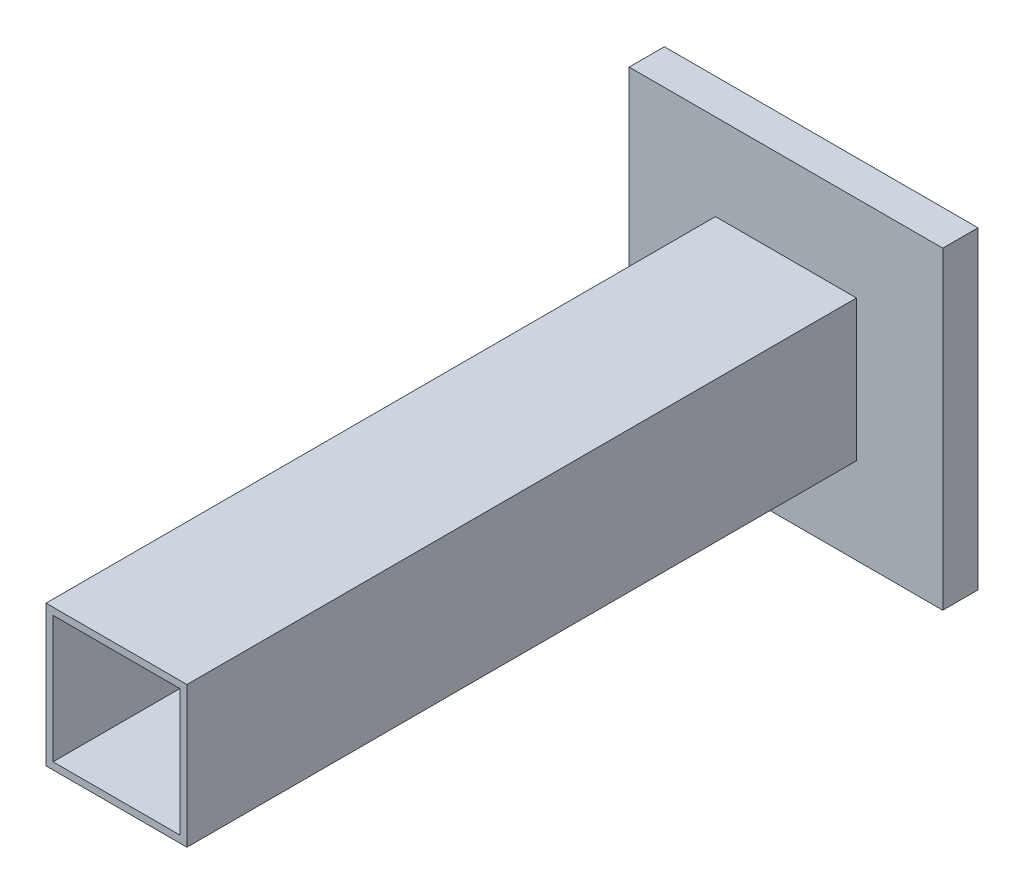
SolidWorks part; units mm, degrees
ref_plane "Front Plane" through (0, 0, 0) normal (0, 0, 1) x (1, 0, 0)
ref_plane "Top Plane" through (0, 0, 0) normal (0, 1, 0) x (1, 0, 0)
ref_plane "Right Plane" through (0, 0, 0) normal (1, 0, 0) x (0, 0, -1)
other "Configuration Table"
sketch "Sketch1" plane through (0, 0, 0) normal (0, 0, 1) x (1, 0, 0)
  line L1 (-222.5, 222.5) -> (222.5, 222.5)
  line L2 (-222.5, 222.5) -> (-222.5, -222.5)
  line L3 (-222.5, -222.5) -> (222.5, -222.5)
  line L4 (222.5, 222.5) -> (222.5, -222.5)
  line L5 (-222.5, 222.5) -> (222.5, -222.5) construction
  line L6 (-222.5, -222.5) -> (222.5, 222.5) construction
  point P0 (0, 0)
  dimension "D1" = 445
  dimension "D2" = 445
extrude "Boss-Extrude1" add sketch "Sketch1" along normal blind 50
sketch "Sketch2" plane through (0, 0, 50) normal (0, 0, 1) x (1, 0, 0)
  line L1 (-100, 100) -> (100, 100)
  line L2 (-100, 100) -> (-100, -100)
  line L3 (-100, -100) -> (100, -100)
  line L4 (100, 100) -> (100, -100)
  line L5 (-100, 100) -> (100, -100) construction
  line L6 (-100, -100) -> (100, 100) construction
  line L7 (-90, 90) -> (90, 90)
  line L8 (-90, 90) -> (-90, -90)
  line L9 (-90, -90) -> (90, -90)
  line L10 (90, 90) -> (90, -90)
  line L11 (-90, 90) -> (90, -90) construction
  line L12 (-90, -90) -> (90, 90) construction
  point P0 (0, 0)
  point P7 (0, 0)
  dimension "D1" = 200
  dimension "D2" = 200
  dimension "D3" = 180
  dimension "D4" = 180
extrude "Boss-Extrude2" add sketch "Sketch2" along normal blind 950
